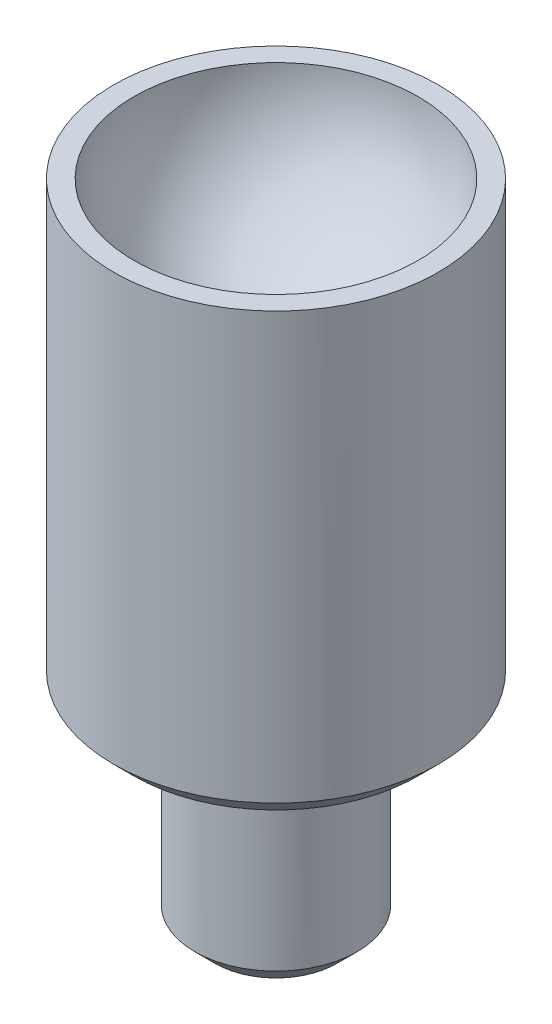
SolidWorks part; units mm, degrees
ref_plane "Front Plane" through (0, 0, 0) normal (0, 0, 1) x (1, 0, 0)
ref_plane "Top Plane" through (0, 0, 0) normal (0, 1, 0) x (1, 0, 0)
ref_plane "Right Plane" through (0, 0, 0) normal (1, 0, 0) x (0, 0, -1)
other "Configuration Table"
sketch "Sketch1" plane through (0, 0, 0) normal (0, 0, 1) x (1, 0, 0)
  line L0 (0, 0) -> (0, 32) construction
  line L1 (-2, 0) -> (-2, 25.2918)
  line L2 (-7, 32) -> (-8, 32)
  line L3 (-8, 32) -> (-8, 10)
  line L5 (-2, 0) -> (-4, 0)
  line L6 (-8, 10) -> (-4, 10)
  line L7 (-4, 10) -> (-4, 0)
  arc A0 (-2, 25.2918) -> (-7, 32) centre (0, 32) cw
  dimension "D6" = 7
  dimension "D7" = 10
  dimension "D1" = 8
  dimension "D2" = 2
  dimension "D3" = 1
  dimension "D4" = 32
  dimension "D5" = 4
revolve "Revolve2" add sketch "Sketch1" angle 360 about L0
cosmetic thread "Cosmetic Thread1" parameters "D2"=7
chamfer "Chamfer1" distance 1 angle 45 2 edges at (0, 10, -8) (0, 0, -4)
